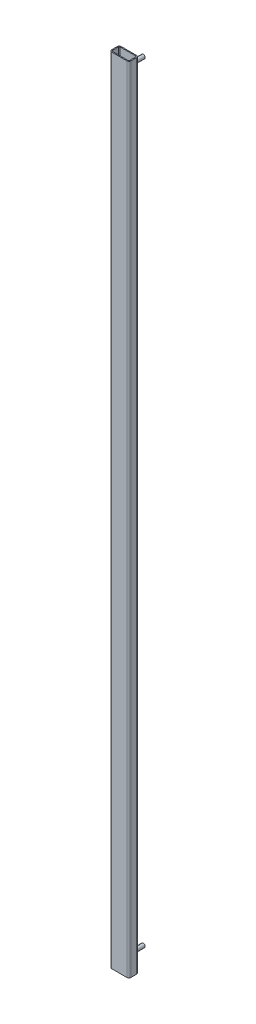
from build123d import *

# Parameters (mm, degrees)
EXTRUDE_1_DEPTH = 1650
SKETCH_2_R      = 4
EXTRUDE_2_DEPTH = 30


with BuildPart() as part:
    # 草图1 → 凸台-拉伸1 (new body)
    with BuildSketch(Plane(origin=(0, 0, 0), x_dir=(1, 0, 0), z_dir=(0, 1, 0))):
        with BuildLine():
            Line((-16, -10), (16, -10))
            ThreePointArc((16, -10), (18.828427125, -8.828427125), (20, -6))
            Line((20, -6), (20, 6))
            ThreePointArc((20, 6), (18.828427125, 8.828427125), (16, 10))
            Line((16, 10), (-16, 10))
            ThreePointArc((-16, 10), (-18.828427125, 8.828427125), (-20, 6))
            Line((-20, 6), (-20, -6))
            ThreePointArc((-20, -6), (-18.828427125, -8.828427125), (-16, -10))
        make_face()
        with BuildLine():
            Line((-16, -8), (16, -8))
            ThreePointArc((16, -8), (17.414213562, -7.414213562), (18, -6))
            Line((18, -6), (18, 6))
            ThreePointArc((18, 6), (17.414213562, 7.414213562), (16, 8))
            Line((16, 8), (-16, 8))
            ThreePointArc((-16, 8), (-17.414213562, 7.414213562), (-18, 6))
            Line((-18, 6), (-18, -6))
            ThreePointArc((-18, -6), (-17.414213562, -7.414213562), (-16, -8))
        make_face(mode=Mode.SUBTRACT)
    extrude(amount=EXTRUDE_1_DEPTH)

    # 草图2 → 凸台-拉伸2 (add)
    with BuildSketch(Plane(origin=(0, 0, -10), x_dir=(-1, 0, 0), z_dir=(0, 0, -1))):
        with Locations(Location((0, 1625, 0), (0, 0, 180))):
            Circle(SKETCH_2_R)
        with Locations(Location((0, 25, 0), (0, 0, 180))):
            Circle(SKETCH_2_R)
    extrude(amount=EXTRUDE_2_DEPTH)


solid = part.part
